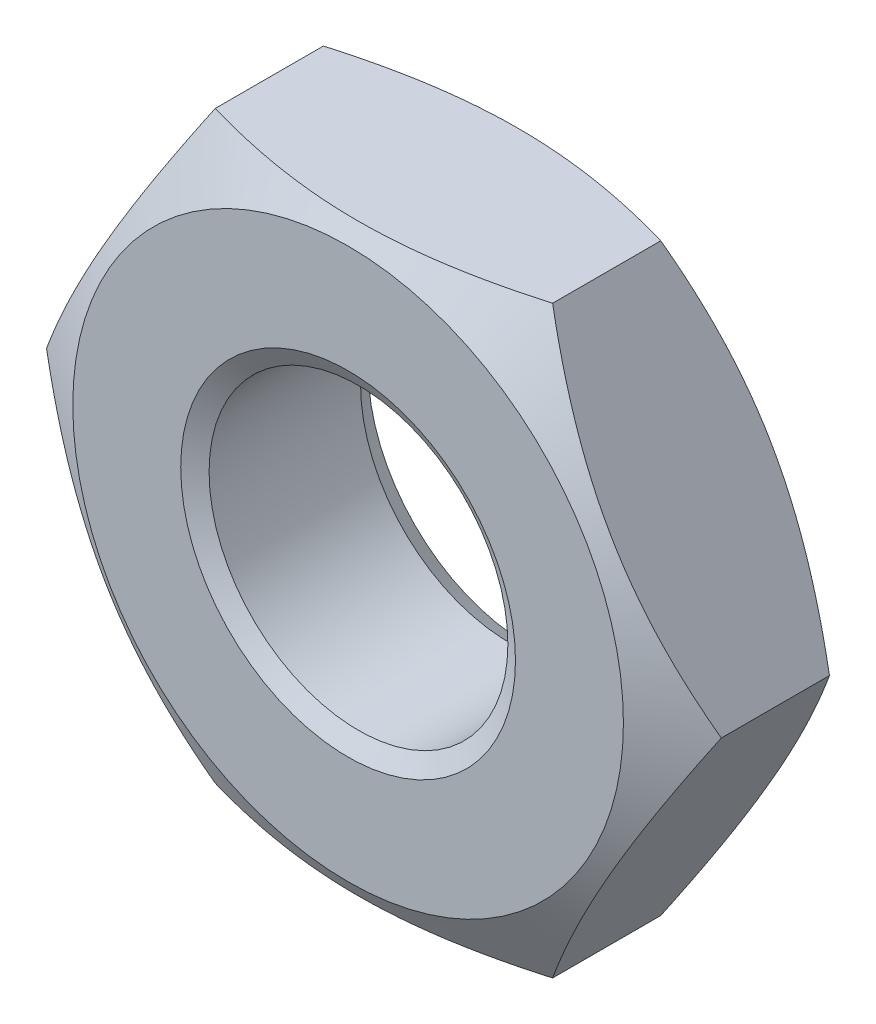
from build123d import *
from OCP.BRepFilletAPI import BRepFilletAPI_MakeChamfer

# Parameters (mm, degrees)
SKETCH1_R        = 3.3235
BASENUT_DEPTH    = 4
ENDCHAMFER_SIZE  = 0.4
ENDCHAMFER_SIZE2 = 0.230940108


with BuildPart() as part:
    # Sketch1 → BaseNut (new body)
    with BuildSketch(Plane.XY):
        Polygon((3.75277675, -6.5), (7.505553499, 0), (3.75277675, 6.5), (-3.75277675, 6.5), (-7.505553499, 0), (-3.75277675, -6.5), align=None)
        Circle(SKETCH1_R, mode=Mode.SUBTRACT)
    extrude(amount=-BASENUT_DEPTH)

    # Sketch2 → Double-Chamfer (revolve, cut)
    with BuildSketch(Plane(origin=(0, 0, 0), x_dir=(1, 0, 0), z_dir=(0, 1, 0))):
        Polygon((-7.505553499, 4), (-6.125, 4), (-7.505553499, 3.202937065), align=None)
        Polygon((-7.505553499, 0.797062935), (-7.505553499, 0), (-6.125, 0), align=None)
    revolve(axis=Axis((0, 0, -3.375940562), (0, 0, 1)), mode=Mode.SUBTRACT)

    # EndChamfer: one chamfer whose edges measure the first distance from different faces: ONE call of the kernel's chamfer builder (chamfer() names one face for all edges)
    endchamfer_edges_1 = [part.edges().sort_by_distance(p)[0] for p in [
        (-3.3235, 0, -4),
    ]]
    endchamfer_side_1 = [part.faces().sort_by_distance(p)[0] for p in [
        (-3.3235, 0, -2),
    ]]
    endchamfer_edges_2 = [part.edges().sort_by_distance(p)[0] for p in [
        (-3.3235, 0, 0),
    ]]
    endchamfer_side_2 = [part.faces().sort_by_distance(p)[0] for p in [
        (5.951758839, 0, 0),
    ]]
    endchamfer = BRepFilletAPI_MakeChamfer(part.part.solid().wrapped)
    for e in endchamfer_edges_1:
        endchamfer.Add(ENDCHAMFER_SIZE, ENDCHAMFER_SIZE2, e.wrapped, endchamfer_side_1[0].wrapped)  # the first distance lies on this face
    for e in endchamfer_edges_2:
        endchamfer.Add(ENDCHAMFER_SIZE, ENDCHAMFER_SIZE2, e.wrapped, endchamfer_side_2[0].wrapped)  # the first distance lies on this face
    add(Compound.cast(endchamfer.Shape()), mode=Mode.REPLACE)


solid = part.part
